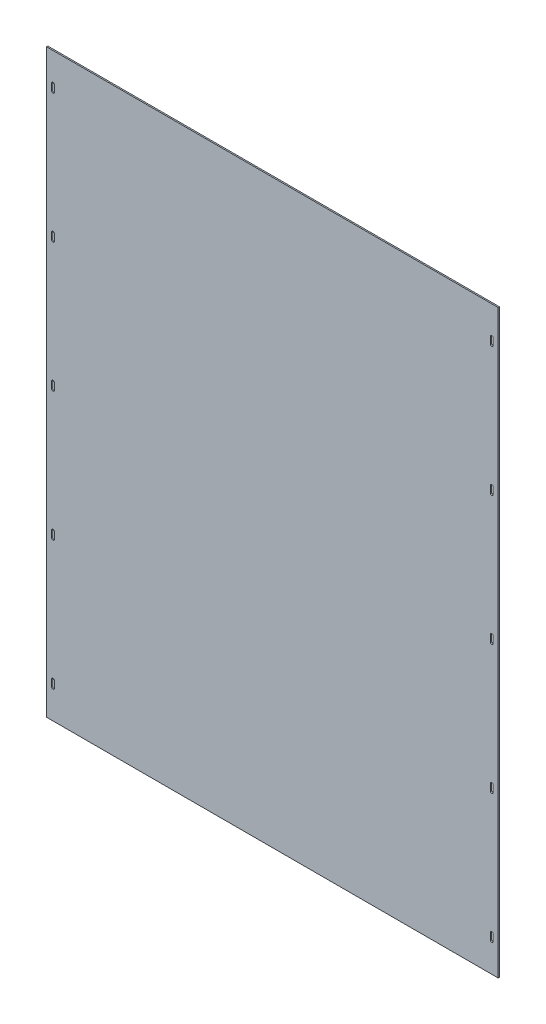
from build123d import *

# Parameters (mm, degrees)
SKETCH_1_W          = 700
SKETCH_1_H          = 900
EXTRUDE_1_DEPTH     = 2
CUT_EXTRUDE_1_DEPTH = 10


with BuildPart() as part:
    # 草图1 → 凸台-拉伸1 (new body)
    with BuildSketch(Plane.XY):
        Rectangle(SKETCH_1_W, SKETCH_1_H)
    extrude(amount=EXTRUDE_1_DEPTH)

    # 草图2 → 切除-拉伸1 (cut)
    with BuildSketch(Plane.XY.offset(2)):
        with BuildLine():
            Line((-337.75, 405), (-337.75, 395))
            ThreePointArc((-337.75, 395), (-340, 392.75), (-342.25, 395))
            Line((-342.25, 395), (-342.25, 405))
            ThreePointArc((-342.25, 405), (-340, 407.25), (-337.75, 405))
        make_face()
        with BuildLine():
            Line((337.75, 405), (337.75, 395))
            ThreePointArc((337.75, 395), (340, 392.75), (342.25, 395))
            Line((342.25, 395), (342.25, 405))
            ThreePointArc((342.25, 405), (340, 407.25), (337.75, 405))
        make_face()
        with BuildLine():
            Line((-342.25, 195), (-342.25, 205))
            ThreePointArc((-342.25, 205), (-340, 207.25), (-337.75, 205))
            Line((-337.75, 205), (-337.75, 195))
            ThreePointArc((-337.75, 195), (-340, 192.75), (-342.25, 195))
        make_face()
        with BuildLine():
            Line((-342.25, -5), (-342.25, 5))
            ThreePointArc((-342.25, 5), (-340, 7.25), (-337.75, 5))
            Line((-337.75, 5), (-337.75, -5))
            ThreePointArc((-337.75, -5), (-340, -7.25), (-342.25, -5))
        make_face()
        with BuildLine():
            Line((342.25, 195), (342.25, 205))
            ThreePointArc((342.25, 205), (340, 207.25), (337.75, 205))
            Line((337.75, 205), (337.75, 195))
            ThreePointArc((337.75, 195), (340, 192.75), (342.25, 195))
        make_face()
        with BuildLine():
            Line((342.25, -5), (342.25, 5))
            ThreePointArc((342.25, 5), (340, 7.25), (337.75, 5))
            Line((337.75, 5), (337.75, -5))
            ThreePointArc((337.75, -5), (340, -7.25), (342.25, -5))
        make_face()
        with BuildLine():
            Line((-342.25, 605), (-342.25, 595))
            ThreePointArc((-342.25, 595), (-340, 592.75), (-337.75, 595))
            Line((-337.75, 595), (-337.75, 605))
            ThreePointArc((-337.75, 605), (-340, 607.25), (-342.25, 605))
        make_face()
        with BuildLine():
            Line((342.25, 605), (342.25, 595))
            ThreePointArc((342.25, 595), (340, 592.75), (337.75, 595))
            Line((337.75, 595), (337.75, 605))
            ThreePointArc((337.75, 605), (340, 607.25), (342.25, 605))
        make_face()
        with BuildLine():
            Line((342.25, -195), (342.25, -205))
            ThreePointArc((342.25, -205), (340, -207.25), (337.75, -205))
            Line((337.75, -205), (337.75, -195))
            ThreePointArc((337.75, -195), (340, -192.75), (342.25, -195))
        make_face()
        with BuildLine():
            Line((-342.25, -195), (-342.25, -205))
            ThreePointArc((-342.25, -205), (-340, -207.25), (-337.75, -205))
            Line((-337.75, -205), (-337.75, -195))
            ThreePointArc((-337.75, -195), (-340, -192.75), (-342.25, -195))
        make_face()
        with BuildLine():
            Line((337.75, -405), (337.75, -395))
            ThreePointArc((337.75, -395), (340, -392.75), (342.25, -395))
            Line((342.25, -395), (342.25, -405))
            ThreePointArc((342.25, -405), (340, -407.25), (337.75, -405))
        make_face()
        with BuildLine():
            Line((-337.75, -405), (-337.75, -395))
            ThreePointArc((-337.75, -395), (-340, -392.75), (-342.25, -395))
            Line((-342.25, -395), (-342.25, -405))
            ThreePointArc((-342.25, -405), (-340, -407.25), (-337.75, -405))
        make_face()
    extrude(amount=-CUT_EXTRUDE_1_DEPTH, mode=Mode.SUBTRACT)


solid = part.part
